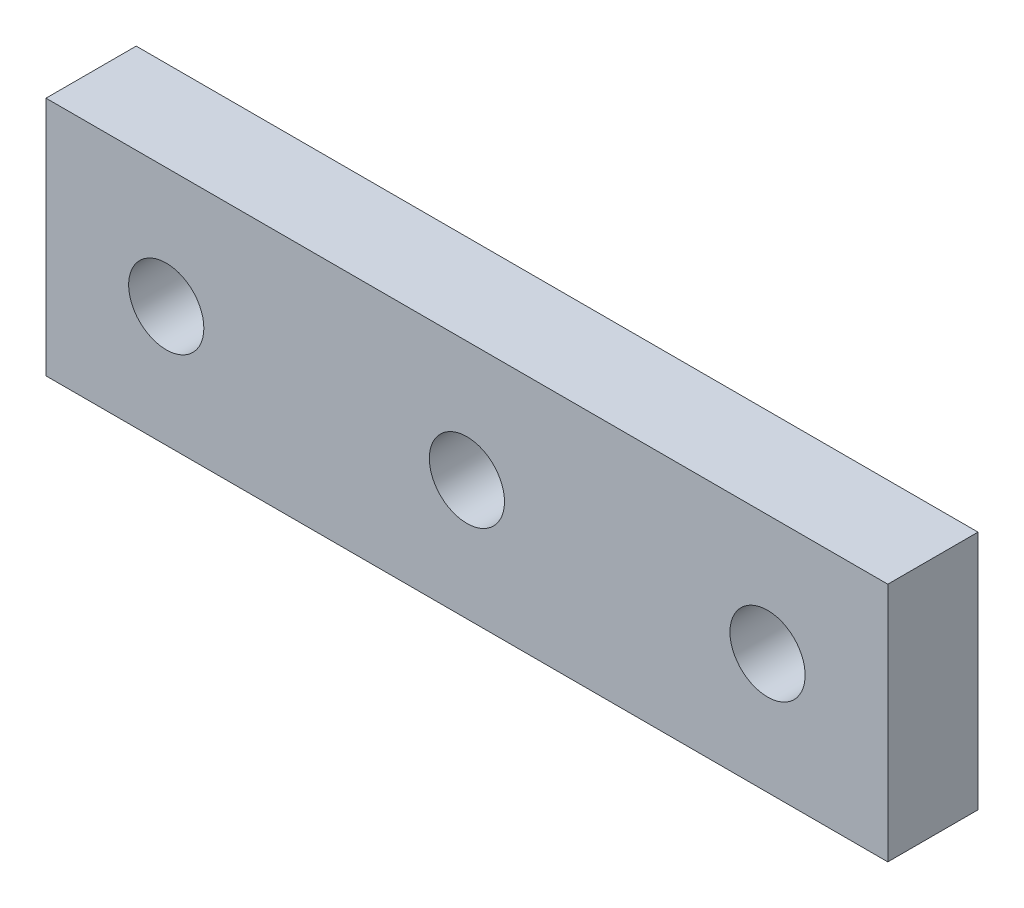
SolidWorks part; units mm, degrees
material "304"
ref_plane "Front Plane" through (0, 0, 0) normal (0, 0, 1) x (1, 0, 0)
ref_plane "Top Plane" through (0, 0, 0) normal (0, 1, 0) x (1, 0, 0)
ref_plane "Right Plane" through (0, 0, 0) normal (1, 0, 0) x (0, 0, -1)
sketch "Sketch1" plane through (0, 0, 0) normal (0, 0, 1) x (1, 0, 0)
  line L0 (0, -4) -> (28, -4) construction
  line L1 (0, 0) -> (28, 0)
  line L2 (0, 0) -> (0, -8)
  line L3 (0, -8) -> (28, -8)
  line L4 (28, 0) -> (28, -8)
  line L5 (14, 0) -> (14, -8) construction
  circle A0 centre (4, -4) radius 1.25
  circle A1 centre (24, -4) radius 1.25
  dimension "D3" = 10
  dimension "D4" = 2.5
  dimension "D1" = 28
  dimension "D2" = 8
extrude "Boss-Extrude1" add sketch "Sketch1" along normal blind 3
hole_wizard "M3 Tapped Hole6" positions "3DSketch2" profile "Sketch3" tap size "M3" standard "GB"
sketch3d "3DSketch2"
  line L0 (4, -4, 3) -> (4, -4, 0) construction
  line L1 (24, -4, 3) -> (24, -4, 0) construction
  point P0 (4, -4, 3)
  point P4 (24, -4, 3)
sketch "Sketch3" plane through (4, -4, 3) normal (1, 0, 0) x (0, -1, 0)
  line L0 (0, 0) -> (0, 8.2511)
  line L1 (0, 8.2511) -> (1.25, 7.5)
  line L2 (1.25, 7.5) -> (1.25, 0)
  line L5 (1.25, 0) -> (0, 0)
  line L10 (0, 8.2511) -> (-1.25, 7.5) construction
  line L11 (0, -6.35) -> (0, 107.95) construction
  dimension "螺纹孔钻头直径" = 2.5
  dimension "螺纹孔钻头深度" = 7.5
  dimension "导头角度" = 118
cosmetic thread "Cosmetic Thread3" parameters "D1"=3, "D2"=3
cosmetic thread "Cosmetic Thread4" parameters "D1"=3, "D2"=3
sketch "Sketch4" plane through (0, 0, 3) normal (0, 0, 1) x (1, 0, 0)
  line L0 (14, 0) -> (14, -8) construction
  line L1 (28, 0) -> (0, 0) construction
  line L2 (0, -8) -> (28, -8) construction
  circle A0 centre (14, -4) radius 1.5
  dimension "D1" = 3
hole_wizard "M3 Tapped Hole1" positions "3DSketch3" profile "Sketch5" tap size "M3" standard "GB"
sketch3d "3DSketch3"
  point P0 (14, -4, 3)
sketch "Sketch5" plane through (14, -4, 3) normal (1, 0, 0) x (0, -1, 0)
  line L0 (0, 0) -> (0, 8.2511)
  line L1 (0, 8.2511) -> (1.25, 7.5)
  line L2 (1.25, 7.5) -> (1.25, 0)
  line L5 (1.25, 0) -> (0, 0)
  line L10 (0, 8.2511) -> (-1.25, 7.5) construction
  line L11 (0, -6.35) -> (0, 107.95) construction
  dimension "螺纹孔钻头直径" = 2.5
  dimension "螺纹孔钻头深度" = 7.5
  dimension "导头角度" = 118
cosmetic thread "Cosmetic Thread5" parameters "D1"=5, "D2"=3
